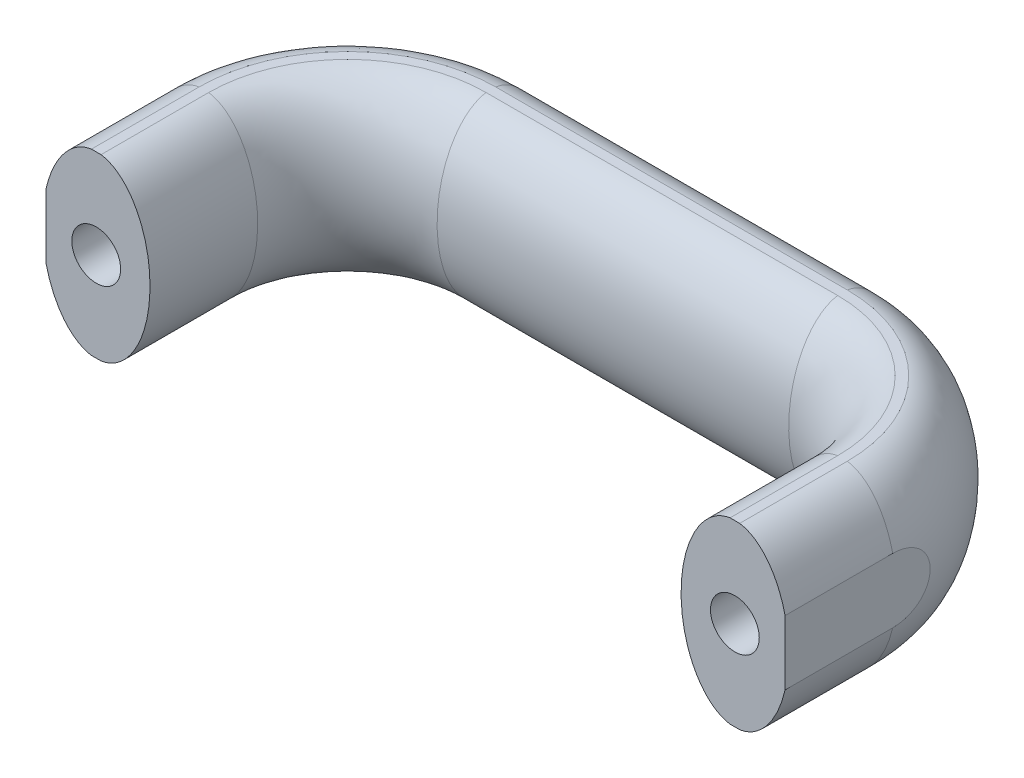
SolidWorks part; units mm, degrees
ref_plane "Front Plane" through (0, 0, 0) normal (0, 0, 1) x (1, 0, 0)
ref_plane "Top Plane" through (0, 0, 0) normal (0, 1, 0) x (1, 0, 0)
ref_plane "Right Plane" through (0, 0, 0) normal (1, 0, 0) x (0, 0, -1)
sketch "Sketch2" plane through (0, 0, 0) normal (0, 0, 1) x (1, 0, 0)
  ellipse E0 centre (0, 0) end of major axis (0, 12.5) minor radius 7.5
  dimension "D1" = 15
  dimension "D2" = 25
sketch "Sketch3" plane through (0, 0, 0) normal (0, 1, 0) x (1, 0, 0)
  line L2 (0, 0) -> (0, 15)
  line L3 (20, 35) -> (69, 35)
  line L4 (89, 0) -> (89, 15)
  arc A0 (89, 15) -> (69, 35) centre (69, 15) ccw
  arc A1 (0, 15) -> (20, 35) centre (20, 15) cw
  point P7 (89, 35)
  point P10 (0, 35)
  dimension "D3" = 20
  dimension "D1" = 89
  dimension "D2" = 35
  dimension "D4" = 35
sweep "Sweep1" add profiles "Sketch2" path "Sketch3"
hole_wizard "M8 Tapped Hole1" positions "Sketch4" profile "Sketch5" tap size "M8" standard "ISO"
sketch "Sketch4" plane through (0, 0, 0) normal (0, 0, 1) x (1, 0, 0)
  point P0 (0, 0)
  point P3 (89, 0)
  dimension "D1" = 89
sketch "Sketch5" plane through (0, 0, 0) normal (1, 0, 0) x (0, -1, 0)
  line L0 (0, 0) -> (0, 21.7929)
  line L1 (0, 21.7929) -> (3.4, 19.75)
  line L2 (3.4, 19.75) -> (3.4, 0)
  line L5 (3.4, 0) -> (0, 0)
  line L10 (0, 21.7929) -> (-3.4, 19.75) construction
  line L11 (0, -6.35) -> (0, 107.95) construction
  dimension "螺纹孔钻头直径" = 6.8
  dimension "螺纹孔钻头深度" = 19.75
  dimension "导头角度" = 118
cosmetic thread "Hole Thread 2" parameters "D1"=16, "D2"=8
cosmetic thread "Hole Thread 3" parameters "D1"=16, "D2"=8
sketch "Sketch6" plane through (0, 0, 0) normal (0, 0, 1) x (1, 0, 0)
  line L0 (44.5, -12.5) -> (44.5, 12.5) construction
  line L1 (-7, -12.45) -> (96, -12.45)
  line L2 (-7, -12.45) -> (-7, 12.45)
  line L3 (-7, 12.45) -> (96, 12.45)
  line L4 (96, -12.45) -> (96, 12.45)
  line L5 (-7, -12.45) -> (96, 12.45) construction
  line L6 (-7, 12.45) -> (96, -12.45) construction
  line L7 (20, -12.5) -> (69, -12.5) construction
  line L8 (69, 12.5) -> (20, 12.5) construction
  line L9 (44.5, 12.5) -> (-7.5, 0) construction
  line L10 (-7.5, 0) -> (96.5, 0) construction
  ellipse E0 centre (0, 0) end of major axis (0, 12.5) minor radius 7.5 construction
  ellipse E1 centre (89, 0) end of major axis (89, 12.5) minor radius 7.5 construction
  point P0 (44.5, 0)
  dimension "D1" = 103
  dimension "D2" = 24.9
extrude "Cut-Extrude-Thin1" cut sketch "Sketch6" against normal through all thin
